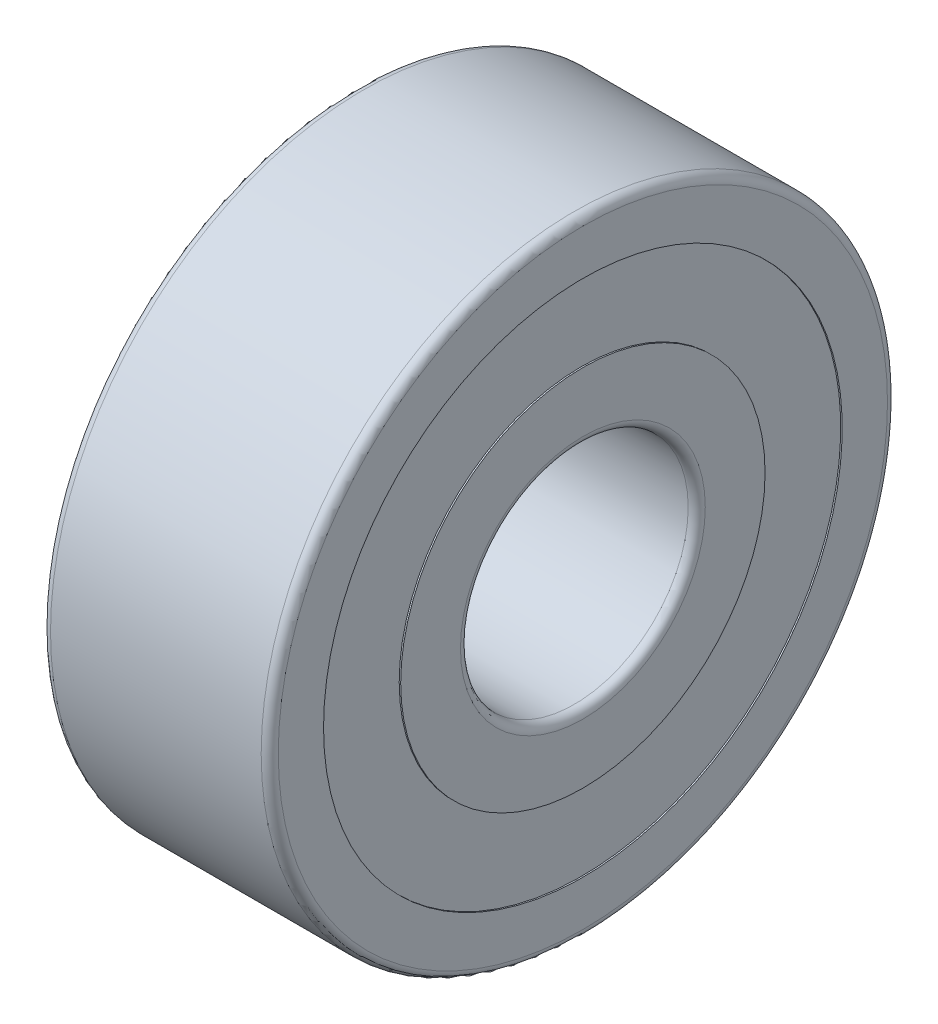
from build123d import *


with BuildPart() as part:
    # 草图1 → 旋转1 (revolve)
    with BuildSketch(Plane.XY, mode=Mode.PRIVATE) as revolve_1_sk:
        with BuildLine():
            Line((0, 5.35), (0, 4.555))
            Line((0, 4.555), (0.026, 4.555))
            Line((0.026, 4.555), (0.026, 3.2))
            Line((0.026, 3.2), (0, 3.2))
            Line((0, 3.2), (0, 2.15))
            ThreePointArc((0, 2.15), (0.043933983, 2.043933983), (0.15, 2))
            Line((0.15, 2), (3.85, 2))
            ThreePointArc((3.85, 2), (3.956066017, 2.043933983), (4, 2.15))
            Line((4, 2.15), (4, 3.2))
            Line((4, 3.2), (3.974, 3.2))
            Line((3.974, 3.2), (3.974, 4.555))
            Line((3.974, 4.555), (4, 4.555))
            Line((4, 4.555), (4, 5.35))
            ThreePointArc((4, 5.35), (3.956066017, 5.456066017), (3.85, 5.5))
            Line((3.85, 5.5), (0.15, 5.5))
            ThreePointArc((0.15, 5.5), (0.043933983, 5.456066017), (0, 5.35))
        make_face()
    revolve(revolve_1_sk.sketch.rotate(Axis((3.85, 0, 0), (-1, 0, 0)), 270), axis=Axis((3.85, 0, 0), (-1, 0, 0)))


solid = part.part
